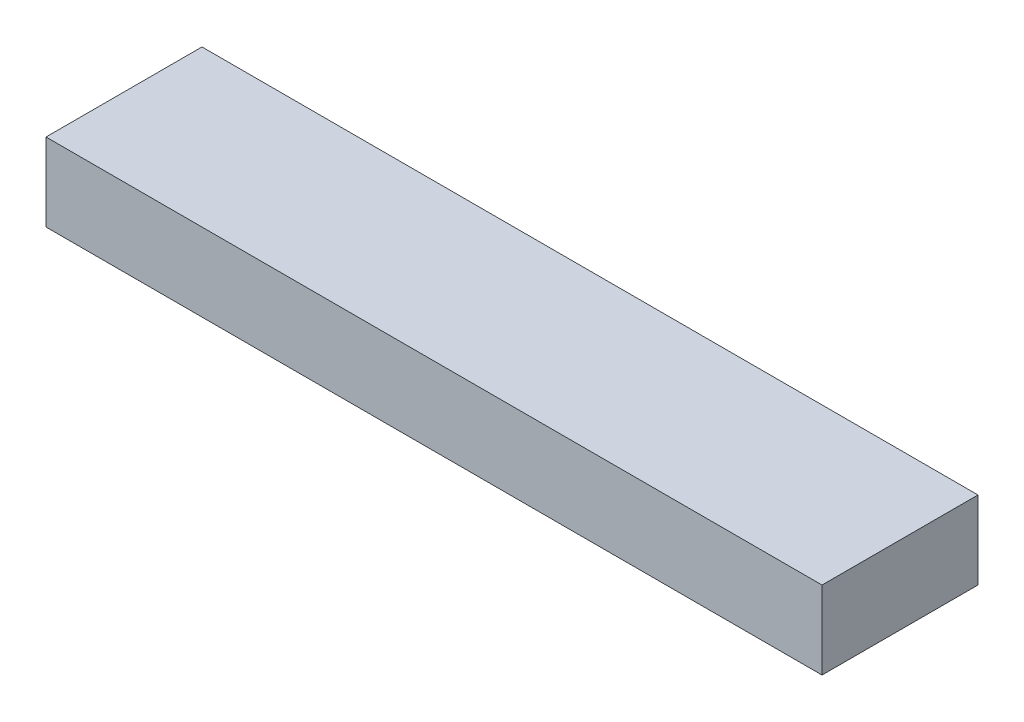
from build123d import *

# Parameters (mm, degrees)
SKETCH1_W           = 199
SKETCH1_H           = 40
BOSS_EXTRUDE1_DEPTH = 20


with BuildPart() as part:
    # Sketch1 → Boss-Extrude1 (new body)
    with BuildSketch(Plane(origin=(0, 0, 0), x_dir=(1, 0, 0), z_dir=(0, 1, 0))):
        with Locations((99.5, 20)):
            Rectangle(SKETCH1_W, SKETCH1_H)
    extrude(amount=BOSS_EXTRUDE1_DEPTH)


solid = part.part
